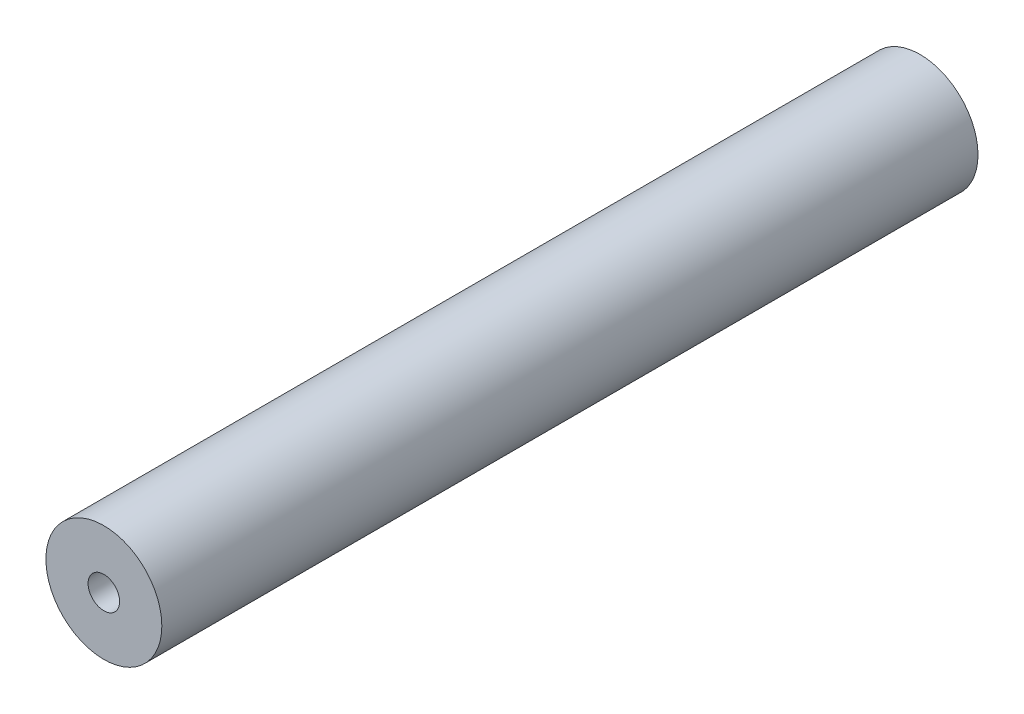
SolidWorks part; units mm, degrees
ref_plane "前视基准面" through (0, 0, 0) normal (0, 0, 1) x (1, 0, 0)
ref_plane "上视基准面" through (0, 0, 0) normal (0, 1, 0) x (1, 0, 0)
ref_plane "右视基准面" through (0, 0, 0) normal (1, 0, 0) x (0, 0, -1)
sketch "草图1" plane through (0, 0, 0) normal (0, 0, 1) x (1, 0, 0)
  circle A0 centre (0, 0) radius 12.5
  dimension "D1" = 25
extrude "凸台-拉伸1" add sketch "草图1" along normal blind 176
hole_wizard "M8 螺纹孔1" positions "草图2" profile "草图3" tap size "M8" standard "GB"
sketch "草图2" plane through (0, 0, 0) normal (0, 0, -1) x (-1, 0, 0)
  point P0 (0, 0)
sketch "草图3" plane through (0, 0, 0) normal (1, 0, 0) x (0, 1, 0)
  line L0 (0, 0) -> (0, 21.7929)
  line L1 (0, 21.7929) -> (3.4, 19.75)
  line L2 (3.4, 19.75) -> (3.4, 0)
  line L5 (3.4, 0) -> (0, 0)
  line L10 (0, 21.7929) -> (-3.4, 19.75) construction
  line L11 (0, -6.35) -> (0, 107.95) construction
  dimension "螺纹孔钻头直径" = 6.8
  dimension "螺纹孔钻头深度" = 19.75
  dimension "导头角度" = 118
cosmetic thread "孔螺蚊线1" parameters "D1"=16, "D2"=8
hole_wizard "M8 螺纹孔2" positions "草图4" profile "草图5" tap size "M8" standard "GB"
sketch "草图4" plane through (0, 0, 176) normal (0, 0, 1) x (1, 0, 0)
  point P0 (0, 0)
sketch "草图5" plane through (0, 0, 176) normal (1, 0, 0) x (0, -1, 0)
  line L0 (0, 0) -> (0, 21.7929)
  line L1 (0, 21.7929) -> (3.4, 19.75)
  line L2 (3.4, 19.75) -> (3.4, 0)
  line L5 (3.4, 0) -> (0, 0)
  line L10 (0, 21.7929) -> (-3.4, 19.75) construction
  line L11 (0, -6.35) -> (0, 107.95) construction
  dimension "螺纹孔钻头直径" = 6.8
  dimension "螺纹孔钻头深度" = 19.75
  dimension "导头角度" = 118
cosmetic thread "孔螺蚊线2" parameters "D1"=16, "D2"=8
